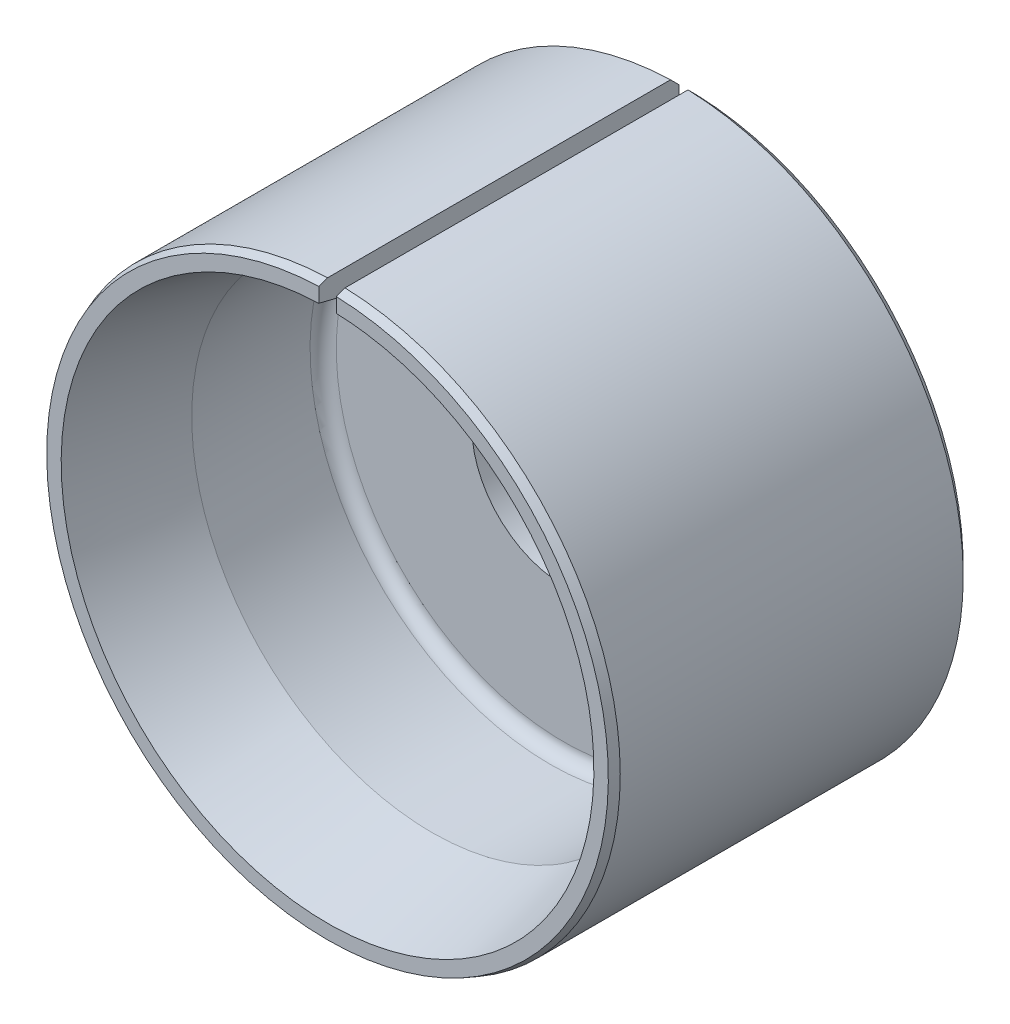
SolidWorks part; units mm, degrees
material "20Mn"
ref_plane "前视基准面" through (0, 0, 0) normal (0, 0, 1) x (1, 0, 0)
ref_plane "上视基准面" through (0, 0, 0) normal (0, 1, 0) x (1, 0, 0)
ref_plane "右视基准面" through (0, 0, 0) normal (1, 0, 0) x (0, 0, -1)
sketch "草图1" plane through (0, 0, 0) normal (0, 0, 1) x (1, 0, 0)
  circle A1 centre (0, 0) radius 32.5
extrude "凸台-拉伸1" add sketch "草图1" along normal blind 41.25
sketch "草图2" plane through (0, 0, 41.25) normal (0, 0, 1) x (1, 0, 0)
  circle A0 centre (0, 0) radius 27.5
extrude "切除-拉伸1" cut sketch "草图2" against normal blind 27
hole_wizard "M24 螺纹孔1" positions "3D草图1" profile "草图3" tap size "M24" standard "GB" end condition through all
sketch3d "3D草图1"
  circle A0 centre (0, 0, 0) radius 32.5 construction
  point P0 (0, 0, 0)
  point P5 (0, 0, 32.5)
sketch "草图3" plane through (0, 0, 0) normal (1, 0, 0) x (0, 1, 0)
  line L0 (0, 0) -> (0, 41.25)
  line L1 (0, 41.25) -> (10.5, 41.25)
  line L2 (10.5, 41.25) -> (10.5, 0)
  line L5 (10.5, 0) -> (0, 0)
  line L11 (0, -6.35) -> (0, 107.95) construction
  dimension "通孔螺纹孔钻头直径" = 21
  dimension "通孔螺纹孔钻头深度" = 41.25
cosmetic thread "孔螺蚊线1" parameters "D2"=24
sketch "草图4" plane through (0, 0, 0) normal (0, 0, -1) x (-1, 0, 0)
  line L0 (0, 0) -> (0, 32.5) construction
  line L2 (-1, 37.0642) -> (1, 37.0642)
  line L3 (-1, 37.0642) -> (-1, -4.5642)
  line L4 (-1, -4.5642) -> (1, -4.5642)
  line L5 (1, 37.0642) -> (1, -4.5642)
  line L6 (-1, 37.0642) -> (1, -4.5642) construction
  line L7 (-1, -4.5642) -> (1, 37.0642) construction
  circle A0 centre (0, 0) radius 32.5 construction
  point P6 (0, 16.25)
  dimension "D1" = 2
extrude "切除-拉伸2" cut sketch "草图4" against normal through all
sketch "草图5" plane through (0, 0, 0) normal (1, 0, 0) x (0, 0, -1)
  line L7 (-41.25, -0.0077) -> (0, 0) construction
  line L8 (-41.25, 32.4846) -> (-41.25, -32.5) construction
  line L11 (-44.25, 27.4818) -> (-29.25, 27.4818)
  line L12 (-41.25, 27.4818) -> (-14.25, 27.4818) construction
  line L13 (-44.25, 27.4818) -> (-44.25, 31.2217)
  line L14 (-44.25, 31.2217) -> (-29.25, 27.4818)
  dimension "D1" = 12
  dimension "D2" = 14
  dimension "D3" = 15
revolve "切除-旋转1" cut sketch "草图5" angle 360 about L7
chamfer "倒角1" distance 1 angle 45 1 edges at (0, -32.5, 0)
chamfer "倒角2" distance 1 angle 20 1 edges at (0, -32.5, 41.25)
fillet "圆角1" radius 1.5 1 edges at (0, -27.5, 14.25)
equation "\"D1@凸台-拉伸1\"=(\"D2@草图1\"-10)*0.75"
equation "\"D1@草图2\"=\"D2@草图1\"-10"
